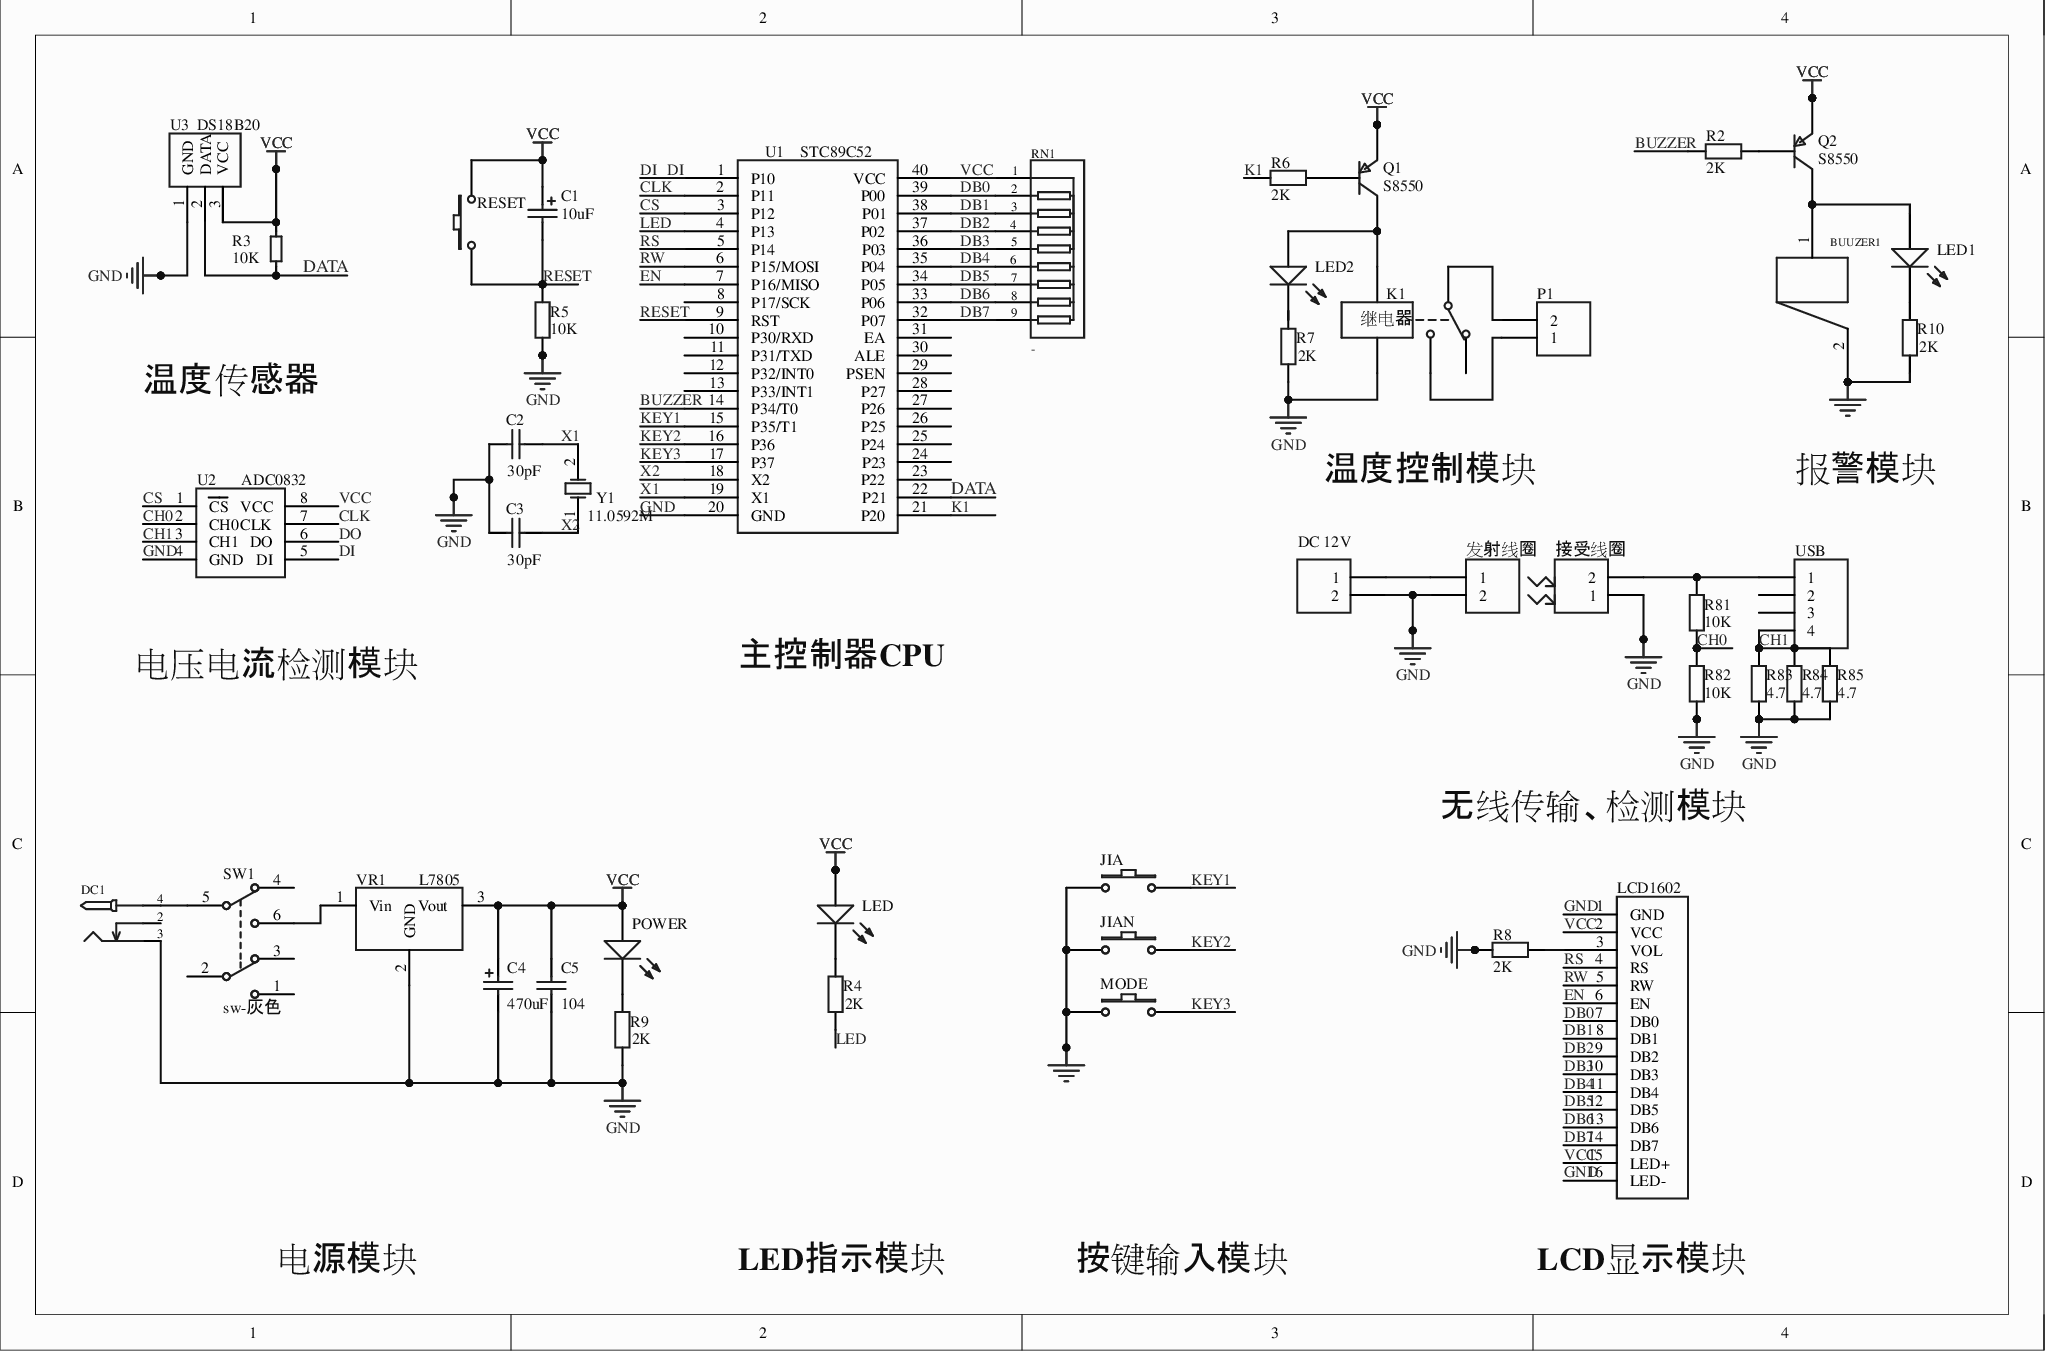
[diagram p0: MISC51120-3.schdoc]
# Altium project MISC51120-2.PrjPcb
1 sheet, 45 parts. Net scope: global (net labels, ports and power ports of the same name join across sheets).
Board file: MISC51120.pcbdoc

## Sheet MISC51120-3.schdoc
size 292 x 193 mm; SheetNumber: 1; SheetTotal: 1; Name: MISC51120

### Parts
BUUZER1  BUZZER  [BUZ-TH_BD12.0-P6.00-D0.9-RD]  (value not drawn)
C1  10uF  [CAP-TH_BD5.0-P2.00-D0.8-FD-10UF50VC110GL]
C2  value 30pF  [CAP-TH_L5.0-W2.5-P5.00-D1.0]  (hidden comment: 18pF)
C3  value 30pF  [CAP-TH_L5.0-W2.5-P5.00-D1.0]  (hidden comment: 18pF)
C4  470uF  [CAP-TH_BD5.0-P2.00-D0.8-FD-10UF50VC110GL]
C5  104  [CAP-TH_L5.0-W2.5-P5.00-D1.0]
DC1  (no value)  [DC-2.0]
DC_12V  Header 2  [HDR-TH_2P-P2.54-V-F]  (value not drawn)
JIA  SW-PB  [KEY-TH_2P-L6.0-W3.9-P6.50]  (value not drawn)
JIAN  SW-PB  [KEY-TH_2P-L6.0-W3.9-P6.50]  (value not drawn)
K1  继电器  [RELAY-TH_G2R-1_C9900014679]
LCD1602  LCD1602  [LCD1602]  (value not drawn)
LED  SI3317-H  [LED_TH-3mm]  (value not drawn)
LED1  SI3317-H  [LED_TH-3mm]  (value not drawn)
LED2  SI3317-H  [LED_TH-3mm]  (value not drawn)
MODE  SW-PB  [KEY-TH_2P-L6.0-W3.9-P6.50]  (value not drawn)
P1  Header 2  [HDR-TH_2P-P2.54-V-F]  (value not drawn)
POWER  SI3317-H  [LED_TH-3mm]  (value not drawn)
Q1  S8550  [TO-92-3_L4.6-W3.6-P1.27-L_1]
Q2  S8550  [TO-92-3_L4.6-W3.6-P1.27-L_1]
R2  value 2K  [Res_1/8W]  (hidden comment: 470)
R3  10K  [Res_1/8W]
R4  value 2K  [Res_1/8W]  (hidden comment: 470)
R5  10K  [Res_1/8W]
R6  value 2K  [Res_1/8W]  (hidden comment: 470)
R7  value 2K  [Res_1/8W]  (hidden comment: 470)
R8  value 2K  [Res_1/8W]  (hidden comment: 470)
R9  value 2K  [Res_1/8W]  (hidden comment: 470)
R10  value 2K  [Res_1/8W]  (hidden comment: 470)
R81  value 10K  [Res_1/8W]  (hidden comment: 470)
R82  value 10K  [Res_1/8W]  (hidden comment: 470)
R83  value 4.7  [Res_1/8W]  (hidden comment: 470)
R84  value 4.7  [Res_1/8W]  (hidden comment: 470)
R85  value 4.7  [Res_1/8W]  (hidden comment: 470)
RESET  SW-PB  [KEY-TH_2P-L6.0-W3.9-P6.50]  (value not drawn)
RN1  -  [RES-ARRAY-TH_9P-P2.54-D1.0]
SW1  sw-灰色  [SW-TH_6P-L8.5-W8.5-P2.54]
U1  STC89C52  [DIP-40_L52.3-W13.9-P2.54-LS15.2-BL-BASE]
U2  ADC0832  [DIP-8_L10.1-W6.3-P2.54-LS7.6-BL]
U3  DS18B20  [TO-92-3_L4.6-W3.6-P1.27-L_1]
USB  Header 4  [HDR-TH_4P-P2.54-V-F]  (value not drawn)
VR1  L7805  [TO-220AB-3_L10.4-W4.6-P2.54-L]
Y1  11.0592M  [HC-49S_L11.0-W4.7-P4.88]
发射线圈  Header 2  [HDR-TH_2P-P2.54-V-F]  (value not drawn)
接受线圈  Header 2  [HDR-TH_2P-P2.54-V-F]  (value not drawn)

### Nets
GND: BUUZER1.2(B) C2.2 C3.2 C4.1 C5.1 DC1.3 DC_12V.2 JIA.1 JIAN.1 K1.5 LCD1602.1(GND) LCD1602.16(LED-) MODE.1 R5.1 R7.1 R8.2 R9.1 R10.1 R82.2 R83.2 R84.2 R85.2 U1.20(GND) U2.4(GND) U3.1(GND) VR1.2(GND) 发射线圈.2 接受线圈.1
VCC: C1.2 C4.2 C5.2 LCD1602.2(VCC) LCD1602.15(LED+) LED.2(A) POWER.2(A) Q1.1(E) Q2.1(E) R3.2 RESET.2 RN1.1 U1.40(VCC) U2.8(VCC) U3.3(VCC) VR1.3(Vout)
BUZZER: R2.2 U1.14(P34/T0)
CH0: R81.2 R82.1 U2.2(CH0)
CH1: R83.1 R84.1 R85.1 U2.3(CH1) USB.4
CLK: U1.2(P11) U2.7(CLK)
CS: U1.3(P12) U2.1(~{CS})
DATA: R3.1 U1.22(P21) U3.2(DATA)
DB0: LCD1602.7(DB0) RN1.2 U1.39(P00)
DB1: LCD1602.8(DB1) RN1.3 U1.38(P01)
DB2: LCD1602.9(DB2) RN1.4 U1.37(P02)
DB3: LCD1602.10(DB3) RN1.5 U1.36(P03)
DB4: LCD1602.11(DB4) RN1.6 U1.35(P04)
DB5: LCD1602.12(DB5) RN1.7 U1.34(P05)
DB6: LCD1602.13(DB6) RN1.8 U1.33(P06)
DB7: LCD1602.14(DB7) RN1.9 U1.32(P07)
DI: U1.1(P10) U2.5(DI)
DO: U2.6(DO)
EN: LCD1602.6(EN) U1.7(P16/MISO)
K1: R6.2 U1.21(P20)
KEY1: JIA.2 U1.15(P35/T1)
KEY2: JIAN.2 U1.16(P36)
KEY3: MODE.2 U1.17(P37)
LED: R4.1 U1.4(P13)
RESET: C1.1 R5.2 RESET.1 U1.9(RST)
RS: LCD1602.4(RS) U1.5(P14)
RW: LCD1602.5(RW) U1.6(P15/MOSI)
X1: C2.1 U1.19(X1) Y1.2(OSC2)
X2: C3.1 U1.18(X2) Y1.1(OSC1)
NetBUUZER1_1: BUUZER1.1(A) LED1.2(A) Q2.3(C)
NetDC1_4: DC1.4 SW1.5(COMMON1)
NetDC_12V_1: DC_12V.1 发射线圈.1
NetK1_1: K1.1 LED2.2(A) Q1.3(C)
NetK1_3: K1.3 P1.1
NetK1_4: K1.4 P1.2
NetLCD1602_3: LCD1602.3(VOL) R8.1
NetLED1_1: LED1.1(K) R10.2
NetLED2_1: LED2.1(K) R7.2
NetLED_1: LED.1(K) R4.2
NetPOWER_1: POWER.1(K) R9.2
NetQ1_2: Q1.2(B) R6.1
NetQ2_2: Q2.2(B) R2.1
NetR81_1: R81.1 USB.1 接受线圈.2
NetSW1_6: SW1.6(NO1) VR1.1(Vin)

Not connected (* = marked no-connect by the designer): DC1 2; K1 2; SW1 1(NO2) 2(COMMON2) 3(NC2) 4(NC1); U1 8(P17/SCK) 10(P30/RXD) 11(P31/TXD) 12(P32/INT0) 13(P33/INT1) 23(P22) 24(P23) 25(P24) 26(P25) 27(P26) 28(P27) 29(PSEN) 30(ALE) 31(EA); USB 2 3

### Notes on the sheet
- 温度传感器
- 温度控制模块
- 报警模块
- 电压电流检测模块
- 主控制器CPU
- 无线传输、检测模块
- 电源模块
- LED指示模块
- 按键输入模块
- (near LCD1602) LCD显示模块

### Library data of the parts
BUUZER1 = BUZZER: Origin Footprint: BUZZER5MM; OriginFootprint 2: BUZZER-5; OriginFootprint 3: BUZZER-8; UniqueId: 023f747ec2b0982d; AddInBom: yes; Device: BUZZER; OriginFootprint 4: BUZZER-5; DesignItemID: BUZZER; LibraryName: *; SymbolName: BUZZER
C1 = Cap Pol2: Polarized Capacitor (Axial); Origin Footprint: C10UF; OriginFootprint 2: CAPPA14.05-10.5x6.3; OriginFootprint 3: CAPPA23.6-18.5x8.5; OriginFootprint 4: CAPPA31.6-26.5x12.5; OriginFootprint 5: CAPPA35.6-30.5x18.5; OriginFootprint 6: CAPPA46.1-41x21.5; OriginFootprint 7: C254DIP; OriginFootprint 8: CAPC4532L; OriginFootprint 9: CAPC5750L; OriginFootprint 10: 7343D; OriginFootprint 12: C; OriginFootprint 14: CAPC2012L; OriginFootprint 15: CAPC3225N; OriginFootprint 16: CAPC3216L; OriginFootprint 19: A-3216; OriginFootprint 21: LED-3MM; UniqueId: b4693cfd16d534cd; AddInBom: yes; Device: Cap Pol2; Published: 8-Jun-2000; LatestRevisionDate: 17-Jul-2002; LatestRevisionNote: Re-released for DXP Platform.; PackageReference: POLAR0.8; Value: 10uF; OriginFootprint 11: 7343D; OriginFootprint 13: 7343D; OriginFootprint 17: C; OriginFootprint 18: C254DIP; OriginFootprint 20: C254DIP; DesignItemID: Cap Pol2; LibraryName: Miscellaneous Devices; SymbolName: Cap Pol2; Publisher: Altium Limited
C2 = Cap: Capacitor; Origin Footprint: C0.1UF; OriginFootprint 2: CAPR2.54-5.1x3.2; OriginFootprint 3: CAPR5.08-7.8x3.2; OriginFootprint 4: C0603; OriginFootprint 5: 2PIN; OriginFootprint 6: HDR1X2; UniqueId: a2c5d49bc5dde298; OriginFootprint 7: C1202; OriginFootprint 9: R0805; AddInBom: yes; Device: Cap; Published: 8-Jun-2000; LatestRevisionDate: 17-Jul-2002; LatestRevisionNote: Re-released for DXP Platform.; PackageReference: RAD-0.3; DesignItemID: Cap; LibraryName: Miscellaneous Devices; SymbolName: Cap; OriginFootprint 8: C0603; OriginFootprint 10: 2PIN; OriginFootprint 11: HDR1X2; Publisher: Altium Limited
C3 = Cap: Capacitor; Origin Footprint: C0.1UF; OriginFootprint 2: CAPR2.54-5.1x3.2; OriginFootprint 3: CAPR5.08-7.8x3.2; OriginFootprint 4: C0603; OriginFootprint 5: 2PIN; OriginFootprint 6: HDR1X2; UniqueId: cc82bf2c2e22e605; OriginFootprint 7: C1202; OriginFootprint 9: R0805; AddInBom: yes; Device: Cap; Published: 8-Jun-2000; LatestRevisionDate: 17-Jul-2002; LatestRevisionNote: Re-released for DXP Platform.; PackageReference: RAD-0.3; DesignItemID: Cap; LibraryName: Miscellaneous Devices; SymbolName: Cap; OriginFootprint 8: C0603; OriginFootprint 10: 2PIN; OriginFootprint 11: HDR1X2; Publisher: Altium Limited
C4 = Cap Pol2: Polarized Capacitor (Axial); Origin Footprint: C470UF; OriginFootprint 2: CAPPA14.05-10.5x6.3; OriginFootprint 3: CAPPA23.6-18.5x8.5; OriginFootprint 4: CAPPA31.6-26.5x12.5; OriginFootprint 5: CAPPA35.6-30.5x18.5; OriginFootprint 6: CAPPA46.1-41x21.5; OriginFootprint 7: C254DIP; OriginFootprint 8: CAPC4532L; OriginFootprint 9: CAPC5750L; OriginFootprint 10: 7343D; OriginFootprint 12: C; OriginFootprint 14: CAPC2012L; OriginFootprint 15: CAPC3225N; OriginFootprint 16: CAPC3216L; OriginFootprint 19: C12*8; UniqueId: 3a68d3ddabf48558; AddInBom: yes; Device: Cap Pol2; Published: 8-Jun-2000; LatestRevisionDate: 17-Jul-2002; LatestRevisionNote: Re-released for DXP Platform.; PackageReference: POLAR0.8; Value: 470uF; OriginFootprint 11: 7343D; OriginFootprint 13: 7343D; OriginFootprint 17: C; OriginFootprint 18: C254DIP; DesignItemID: Cap Pol2; LibraryName: Miscellaneous Devices; SymbolName: Cap Pol2; Publisher: Altium Limited
C5 = Cap: Capacitor; Origin Footprint: C0.1UF; OriginFootprint 2: CAPR2.54-5.1x3.2; OriginFootprint 3: CAPR5.08-7.8x3.2; OriginFootprint 5: C0805; OriginFootprint 6: CAPC2012L; OriginFootprint 7: C1202; OriginFootprint 8: C0603; OriginFootprint 9: R0805; OriginFootprint 10: 2PIN; OriginFootprint 11: HDR1X2; UniqueId: ddba3c46cf8b8e66; AddInBom: yes; Device: Cap; Published: 8-Jun-2000; LatestRevisionDate: 17-Jul-2002; LatestRevisionNote: Re-released for DXP Platform.; PackageReference: RAD-0.3; Value: 104; OriginFootprint 4: 104; DesignItemID: Cap; LibraryName: Miscellaneous Devices; SymbolName: Cap; Publisher: Altium Limited
DC1 = DC-005_2.0: Symbol: DC电源接口; ConvertToPcb: yes; ModelId: f5f20b8a2308479b936ba3c2698865bb0819f05c4eef4c71ace90d822a990e87; ModelName: DC-IN-TH_DC-5520-1; ModelTransform: 372.05,551.18,582.68,90,0,0,137.8,0,-149.61; Device: DC-005_2.0; AddInBom: yes; Supplier Footprint: 插件; FootprintName: DC-2.0
DC_12V = Header 2: Header, 2-Pin; Origin Footprint: HDR1X2; UniqueId: 72eb3ba5b10b2aeb; AddInBom: yes; Device: Header 2; LatestRevisionDate: 17-Jul-2002; LatestRevisionNote: Re-released for DXP Platform.; DesignItemID: Header 2; LibraryName: Miscellaneous Connectors; SymbolName: Header 2; Publisher: Altium Limited
JIA = SW-PB_1: Switch; Origin Footprint: KEY-DIP; UniqueId: 1ca8959cbebd1375; AddInBom: yes; Device: SW-PB_1; Published: 24-Mar-1999; LatestRevisionDate: 17-Jul-2002; LatestRevisionNote: Re-released for DXP Platform.; PackageReference: SPST-2; DesignItemID: SW-PB; LibraryName: *; SymbolName: SW-PB; Publisher: Altium Limited
JIAN = SW-PB_2: Switch; Origin Footprint: KEY-DIP; UniqueId: 34aa0427747adae0; AddInBom: yes; Device: SW-PB_2; Published: 24-Mar-1999; LatestRevisionDate: 17-Jul-2002; LatestRevisionNote: Re-released for DXP Platform.; PackageReference: SPST-2; DesignItemID: SW-PB; LibraryName: *; SymbolName: SW-PB; Publisher: Altium Limited
K1 = Relay-SPDT: Single-Pole Dual-Throw Relay; Origin Footprint: JDQ; Symbol: Relay-SPDT_1; UniqueId: 4da78d22c74f1c2b; AddInBom: yes; Device: Relay-SPDT; Published: 24-Mar-1999; LatestRevisionDate: 17-Jul-2002; LatestRevisionNote: Re-released for DXP Platform.; PackageReference: MODULE5B; DesignItemID: Relay-SPDT; LibraryName: Miscellaneous Devices; Publisher: Altium Limited
LCD1602 = LCD1602: UniqueId: 16bac2fe75c02026; AddInBom: yes; ModelId: f9d832f46a914cadb50fc4d4cefd2517; Device: LCD1602; Origin Footprint: LCD1602; DesignItemID: LCD1602; LibraryName: Schlib1; SymbolName: LCD1602; FootprintName: LCD1602; ModelName: LCD1602
LED = LED0_1: Typical INFRARED GaAs LED; Origin Footprint: LED-R; OriginFootprint 2: D; OriginFootprint 4: VF; OriginFootprint 5: PIN2-D; OriginFootprint 6: LED-5MM; UniqueId: 6e48e3d381ac224f; SymbolName: LED0; AddInBom: yes; Device: LED0_1; Published: 8-Jun-2000; LatestRevisionDate: 08-Jul-2005; LatestRevisionNote: Mech Layer 1 removed.; PackageReference: LED-0; OriginFootprint 3: D; DesignItemID: LED0; LibraryName: Miscellaneous Devices; Publisher: Altium Limited
LED1 = LED0_1: Typical INFRARED GaAs LED; Origin Footprint: LED-R; OriginFootprint 2: D; OriginFootprint 4: VF; UniqueId: 7a65b453ee5a9ec2; SymbolName: LED0; OriginFootprint 5: PIN2-D; OriginFootprint 6: LED-5MM; AddInBom: yes; Device: LED0_1; Published: 8-Jun-2000; LatestRevisionDate: 08-Jul-2005; LatestRevisionNote: Mech Layer 1 removed.; PackageReference: LED-0; OriginFootprint 3: D; DesignItemID: LED0; LibraryName: *; Publisher: Altium Limited
LED2 = LED0_1: Typical INFRARED GaAs LED; Origin Footprint: LED-R; OriginFootprint 2: D; OriginFootprint 4: VF; OriginFootprint 5: PIN2-D; OriginFootprint 6: LED-5MM; UniqueId: 48c2d4982f4ec99a; SymbolName: LED0; AddInBom: yes; Device: LED0_1; Published: 8-Jun-2000; LatestRevisionDate: 08-Jul-2005; LatestRevisionNote: Mech Layer 1 removed.; PackageReference: LED-0; OriginFootprint 3: D; DesignItemID: LED0; LibraryName: Miscellaneous Devices; Publisher: Altium Limited
MODE = SW-PB_3: Switch; Origin Footprint: KEY-DIP; UniqueId: b16f1d7de716d5e8; AddInBom: yes; Device: SW-PB_3; Published: 24-Mar-1999; LatestRevisionDate: 17-Jul-2002; LatestRevisionNote: Re-released for DXP Platform.; PackageReference: SPST-2; DesignItemID: SW-PB; LibraryName: *; SymbolName: SW-PB; Publisher: Altium Limited
P1 = Header 2_3: Header, 2-Pin; Origin Footprint: HDR1X2; UniqueId: c39ee3c861a7b382; AddInBom: yes; Device: Header 2_3; LatestRevisionDate: 17-Jul-2002; LatestRevisionNote: Re-released for DXP Platform.; DesignItemID: Header 2; LibraryName: Miscellaneous Connectors; SymbolName: Header 2; Publisher: Altium Limited
POWER = LED0: Typical INFRARED GaAs LED; Origin Footprint: LED-R; OriginFootprint 2: D; OriginFootprint 4: VF; OriginFootprint 5: PIN2-D; OriginFootprint 6: LED-5MM; UniqueId: c630ca5ef9197c73; AddInBom: yes; Device: LED0; Published: 8-Jun-2000; LatestRevisionDate: 08-Jul-2005; LatestRevisionNote: Mech Layer 1 removed.; PackageReference: LED-0; OriginFootprint 3: D; DesignItemID: LED0; LibraryName: Miscellaneous Devices; SymbolName: LED0; Publisher: Altium Limited
Q1 = 2N3906: PNP General Purpose Amplifier; Origin Footprint: PNP-NPN; OriginFootprint 2: Q-DIP; UniqueId: f76c01de5337d462; AddInBom: yes; Device: 2N3906; Published: 8-Jun-2000; LatestRevisionDate: 15-Jan-2003; LatestRevisionNote: PCB Footprint 'BCY-W3/D4.7' replaced; DatasheetVersion: 1997; PackageVersion: Sep-1998; PackageReference: TO-92A; Code_JEDEC: TO-92A; ComponentLink1Description: Manufacturer Link; ComponentLink1URL: http://www.fairchildsemi.com/; ComponentLink2Description: Datasheet; ComponentLink2URL: http://www.fairchildsemi.com/ds/2N%2F2N3906.pdf; OriginFootprint 3: Q-DIP; DesignItemID: 2N3906; LibraryName: Miscellaneous Devices; SymbolName: 2N3906; Publisher: Altium Limited
Q2 = 2N3906: PNP General Purpose Amplifier; Origin Footprint: PNP-NPN; OriginFootprint 2: Q-DIP; UniqueId: 4c27cd76e8dbac26; AddInBom: yes; Device: 2N3906; Published: 8-Jun-2000; LatestRevisionDate: 15-Jan-2003; LatestRevisionNote: PCB Footprint 'BCY-W3/D4.7' replaced; DatasheetVersion: 1997; PackageVersion: Sep-1998; PackageReference: TO-92A; Code_JEDEC: TO-92A; ComponentLink1Description: Manufacturer Link; ComponentLink1URL: http://www.fairchildsemi.com/; ComponentLink2Description: Datasheet; ComponentLink2URL: http://www.fairchildsemi.com/ds/2N%2F2N3906.pdf; OriginFootprint 3: Q-DIP; DesignItemID: 2N3906; LibraryName: *; SymbolName: 2N3906; Publisher: Altium Limited
R2 = 0805: Resistor; Origin Footprint: AXIAL0.3; OriginFootprint 2: RESC5025L; OriginFootprint 4: RESC2012N; UniqueId: 6f63fc6711cfa315; AddInBom: yes; Device: 0805; Published: 8-Jun-2000; LatestRevisionDate: 17-Jul-2002; LatestRevisionNote: Re-released for DXP Platform.; PackageReference: AXIAL-0.4; OriginFootprint 3: 0805; DesignItemID: 0805; LibraryName: *; SymbolName: 0805; Publisher: Altium Limited
R3 = RES2: Origin Footprint: res400mil; UniqueId: fe89d0632cfce75f; AddInBom: yes; Device: RES2; DesignItemID: RES2; LibraryName: C8051F020最小2; SymbolName: RES2
R4 = Res2: Resistor; Origin Footprint: AXIAL0.3; OriginFootprint 2: R0805; OriginFootprint 3: R0603; OriginFootprint 4: 2PIN; UniqueId: fdc86a4b576d9e98; OriginFootprint 5: R1201; OriginFootprint 6: R1202; AddInBom: yes; Device: Res2; Published: 8-Jun-2000; LatestRevisionDate: 17-Jul-2002; LatestRevisionNote: Re-released for DXP Platform.; PackageReference: AXIAL-0.4; DesignItemID: Res2; LibraryName: Miscellaneous Devices; SymbolName: Res2; OriginFootprint 7: R0603; OriginFootprint 8: 2PIN; Publisher: Altium Limited
R5 = Res2: Resistor; Origin Footprint: AXIAL0.3; OriginFootprint 2: RESC5025L; OriginFootprint 3: 0805; OriginFootprint 4: RESC2012N; OriginFootprint 5: R1201; OriginFootprint 6: R1202; OriginFootprint 7: R0603; OriginFootprint 8: 2PIN; UniqueId: 9cdd622c9eeecfe7; AddInBom: yes; Device: Res2; Published: 8-Jun-2000; LatestRevisionDate: 17-Jul-2002; LatestRevisionNote: Re-released for DXP Platform.; PackageReference: AXIAL-0.4; Value: 10K; DesignItemID: Res2; LibraryName: Miscellaneous Devices; SymbolName: Res2; Publisher: Altium Limited
R6 = Res2_1: Resistor; Origin Footprint: AXIAL0.3; OriginFootprint 2: RESC5025L; OriginFootprint 3: 0805; OriginFootprint 4: RESC2012N; OriginFootprint 5: R1201; OriginFootprint 6: R1202; OriginFootprint 7: R0603; OriginFootprint 8: 2PIN; UniqueId: e06ccd13940482ac; SymbolName: Res2; AddInBom: yes; Device: Res2_1; Published: 8-Jun-2000; LatestRevisionDate: 17-Jul-2002; LatestRevisionNote: Re-released for DXP Platform.; PackageReference: AXIAL-0.4; DesignItemID: Res2; LibraryName: Miscellaneous Devices; Publisher: Altium Limited
R7 = Res2: Resistor; Origin Footprint: AXIAL0.3; OriginFootprint 2: R0805; OriginFootprint 3: R0603; OriginFootprint 4: 2PIN; UniqueId: ba2c6d155e7fd301; OriginFootprint 5: R1201; OriginFootprint 6: R1202; AddInBom: yes; Device: Res2; Published: 8-Jun-2000; LatestRevisionDate: 17-Jul-2002; LatestRevisionNote: Re-released for DXP Platform.; PackageReference: AXIAL-0.4; DesignItemID: Res2; LibraryName: Miscellaneous Devices; SymbolName: Res2; OriginFootprint 7: R0603; OriginFootprint 8: 2PIN; Publisher: Altium Limited
R8 = Res2_1: Resistor; Origin Footprint: AXIAL0.3; OriginFootprint 2: RESC5025L; OriginFootprint 3: 0805; OriginFootprint 4: RESC2012N; OriginFootprint 5: R1201; OriginFootprint 6: R1202; OriginFootprint 7: R0603; OriginFootprint 8: 2PIN; UniqueId: 86d447fa2a9c8586; SymbolName: Res2; AddInBom: yes; Device: Res2_1; Published: 8-Jun-2000; LatestRevisionDate: 17-Jul-2002; LatestRevisionNote: Re-released for DXP Platform.; PackageReference: AXIAL-0.4; DesignItemID: Res2; LibraryName: Miscellaneous Devices; Publisher: Altium Limited
R9 = Res2: Resistor; Origin Footprint: AXIAL0.3; OriginFootprint 2: R0805; OriginFootprint 3: R0603; OriginFootprint 4: 2PIN; UniqueId: 1e1ffada38203b9e; OriginFootprint 5: R1201; OriginFootprint 6: R1202; AddInBom: yes; Device: Res2; Published: 8-Jun-2000; LatestRevisionDate: 17-Jul-2002; LatestRevisionNote: Re-released for DXP Platform.; PackageReference: AXIAL-0.4; DesignItemID: Res2; LibraryName: Miscellaneous Devices; SymbolName: Res2; OriginFootprint 7: R0603; OriginFootprint 8: 2PIN; Publisher: Altium Limited
R10 = Res2: Resistor; Origin Footprint: AXIAL0.3; OriginFootprint 2: R0805; OriginFootprint 3: R0603; OriginFootprint 4: 2PIN; UniqueId: 41bc0941336b1513; OriginFootprint 5: R1201; OriginFootprint 6: R1202; AddInBom: yes; Device: Res2; Published: 8-Jun-2000; LatestRevisionDate: 17-Jul-2002; LatestRevisionNote: Re-released for DXP Platform.; PackageReference: AXIAL-0.4; DesignItemID: Res2; LibraryName: *; SymbolName: Res2; OriginFootprint 7: R0603; OriginFootprint 8: 2PIN; Publisher: Altium Limited
R81 = Res2: Resistor; Origin Footprint: AXIAL0.3; OriginFootprint 2: RESC5025L; OriginFootprint 3: 0805; OriginFootprint 4: RESC2012N; OriginFootprint 5: R1201; OriginFootprint 6: R1202; OriginFootprint 7: R0603; OriginFootprint 8: 2PIN; UniqueId: 3011db0f8b83c791; AddInBom: yes; Device: Res2; Published: 8-Jun-2000; LatestRevisionDate: 17-Jul-2002; LatestRevisionNote: Re-released for DXP Platform.; PackageReference: AXIAL-0.4; DesignItemID: Res2; LibraryName: Miscellaneous Devices; SymbolName: Res2; Publisher: Altium Limited
R82 = Res2: Resistor; Origin Footprint: AXIAL0.3; OriginFootprint 2: RESC5025L; OriginFootprint 3: 0805; OriginFootprint 4: RESC2012N; OriginFootprint 5: R1201; OriginFootprint 6: R1202; OriginFootprint 7: R0603; OriginFootprint 8: 2PIN; UniqueId: cee6f05d4f5da217; AddInBom: yes; Device: Res2; Published: 8-Jun-2000; LatestRevisionDate: 17-Jul-2002; LatestRevisionNote: Re-released for DXP Platform.; PackageReference: AXIAL-0.4; DesignItemID: Res2; LibraryName: Miscellaneous Devices; SymbolName: Res2; Publisher: Altium Limited
R83 = Res2: Resistor; Origin Footprint: AXIAL0.3; OriginFootprint 2: RESC5025L; OriginFootprint 3: 0805; OriginFootprint 4: RESC2012N; OriginFootprint 5: R1201; OriginFootprint 6: R1202; OriginFootprint 7: R0603; OriginFootprint 8: 2PIN; UniqueId: 2def0c7bfd9fbeed; AddInBom: yes; Device: Res2; Published: 8-Jun-2000; LatestRevisionDate: 17-Jul-2002; LatestRevisionNote: Re-released for DXP Platform.; PackageReference: AXIAL-0.4; DesignItemID: Res2; LibraryName: Miscellaneous Devices; SymbolName: Res2; Publisher: Altium Limited
R84 = Res2: Resistor; Origin Footprint: AXIAL0.3; OriginFootprint 2: RESC5025L; OriginFootprint 3: 0805; OriginFootprint 4: RESC2012N; OriginFootprint 5: R1201; OriginFootprint 6: R1202; OriginFootprint 7: R0603; OriginFootprint 8: 2PIN; UniqueId: 4d191c4b38f731f1; AddInBom: yes; Device: Res2; Published: 8-Jun-2000; LatestRevisionDate: 17-Jul-2002; LatestRevisionNote: Re-released for DXP Platform.; PackageReference: AXIAL-0.4; DesignItemID: Res2; LibraryName: Miscellaneous Devices; SymbolName: Res2; Publisher: Altium Limited
R85 = Res2: Resistor; Origin Footprint: AXIAL0.3; OriginFootprint 2: RESC5025L; OriginFootprint 3: 0805; OriginFootprint 4: RESC2012N; OriginFootprint 5: R1201; OriginFootprint 6: R1202; OriginFootprint 7: R0603; OriginFootprint 8: 2PIN; UniqueId: 77dd5bfa062b9469; AddInBom: yes; Device: Res2; Published: 8-Jun-2000; LatestRevisionDate: 17-Jul-2002; LatestRevisionNote: Re-released for DXP Platform.; PackageReference: AXIAL-0.4; DesignItemID: Res2; LibraryName: Miscellaneous Devices; SymbolName: Res2; Publisher: Altium Limited
RESET = SW-PB: Switch; Origin Footprint: KEY-DIP; UniqueId: 21cfdc0312b2838b; AddInBom: yes; Device: SW-PB; Published: 24-Mar-1999; LatestRevisionDate: 17-Jul-2002; LatestRevisionNote: Re-released for DXP Platform.; PackageReference: SPST-2; DesignItemID: SW-PB; LibraryName: Miscellaneous Devices; SymbolName: SW-PB; Publisher: Altium Limited
RN1 = 排阻 10 K 5%: 电阻器数:-;阻值:-;单个元件功率:-;; Symbol: 10 K 5%; 3D Model: d106c67f29e14d8080ba548247a719a10819f05c4eef4c71ace90d822a990e87; 3D Model Transform: 918.1084,118.11,0,0,0,0,0,0,-137.795; AddInBom: yes; ModelName: SIP-9_L22.8-W3.0-H8.5-P2.54; Device: 排阻 10 K 5%; LCSC Part Name: 10KΩ (103) ±5%; Supplier Part: C26615; Manufacturer Part: 排阻 10 K 5%; Supplier Footprint: 插件; JLCPCB Part Class: Extended Part; Supplier: LCSC; Number of Resistors: -; Value: -; Power(Watts): -; Number of Pins: -; ConvertToPcb: yes; FootprintName: RES-ARRAY-TH_9P-P2.54-D1.0
SW1 = sw-灰色: Origin Footprint: DIP6/1; UniqueId: c39dab7994ba8bcb; AddInBom: yes; Device: sw-灰色; DesignItemID: sw-灰色; LibraryName: PERSON_A; SymbolName: sw-灰色
U1 = AT89S52: Origin Footprint: DIP40; UniqueId: 1bdc0ab44f99f92d; AddInBom: yes; Device: AT89S52; DesignItemID: AT89S52; LibraryName: 主控板; SymbolName: AT89S52
U2 = Component_2: Origin Footprint: DIP8; UniqueId: 48f0ae2437312dae; AddInBom: yes; Device: Component_2; DesignItemID: Component_2; LibraryName: Schlib1; SymbolName: Component_2
U3 = DS18B20: Origin Footprint: 18B20; UniqueId: 66797bcd97f4f6c2; AddInBom: yes; Device: DS18B20; DesignItemID: DS18B20; LibraryName: 实验板原理图; SymbolName: DS18B20
USB = Header 4: Header, 4-Pin; Origin Footprint: HDR1X4; UniqueId: 18f7317328dcd701; AddInBom: yes; Device: Header 4; LatestRevisionDate: 17-Jul-2002; LatestRevisionNote: Re-released for DXP Platform.; DesignItemID: Header 4; LibraryName: Miscellaneous Connectors; SymbolName: Header 4; Publisher: Altium Limited
VR1 = 78xx: Origin Footprint: TO-220-1; UniqueId: 8e857b1cff8fa7ed; AddInBom: yes; Device: 78xx; DesignItemID: 78xx; LibraryName: PERSON_A标准; SymbolName: 78xx
Y1 = XTAL: Crystal Oscillator; Origin Footprint: YDIP; OriginFootprint 2: YMHZ; OriginFootprint 3: Y; UniqueId: 9790cc8ece124e27; AddInBom: yes; Device: XTAL; Published: 8-Jun-2000; LatestRevisionDate: 17-Jul-2002; LatestRevisionNote: Re-released for DXP Platform.; PackageReference: R38; DesignItemID: XTAL; LibraryName: Miscellaneous Devices; SymbolName: XTAL; Publisher: Altium Limited
发射线圈 = Header 2_1: Header, 2-Pin; Origin Footprint: HDR1X2; UniqueId: d5b77272221f3065; AddInBom: yes; Device: Header 2_1; LatestRevisionDate: 17-Jul-2002; LatestRevisionNote: Re-released for DXP Platform.; DesignItemID: Header 2; LibraryName: Miscellaneous Connectors; SymbolName: Header 2; Publisher: Altium Limited
接受线圈 = Header 2_2: Header, 2-Pin; Origin Footprint: HDR1X2; UniqueId: 0ea8e72fdaa952f4; AddInBom: yes; Device: Header 2_2; LatestRevisionDate: 17-Jul-2002; LatestRevisionNote: Re-released for DXP Platform.; DesignItemID: Header 2; LibraryName: Miscellaneous Connectors; SymbolName: Header 2; Publisher: Altium Limited